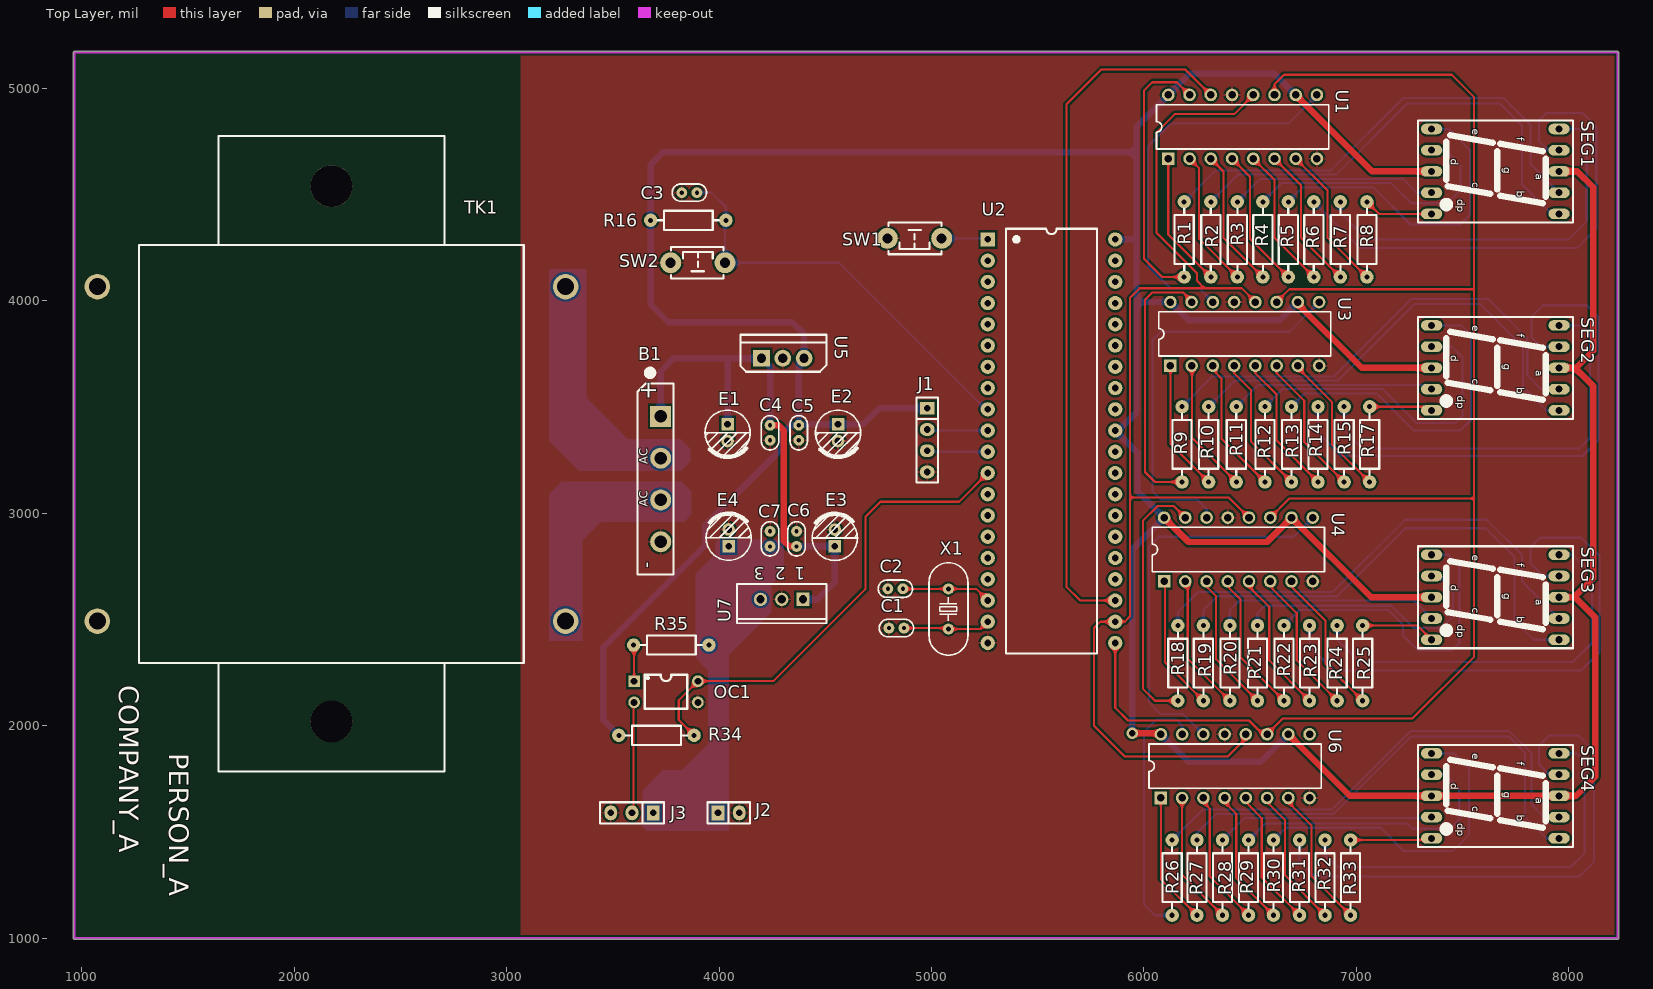
[diagram p0: Top Layer view]
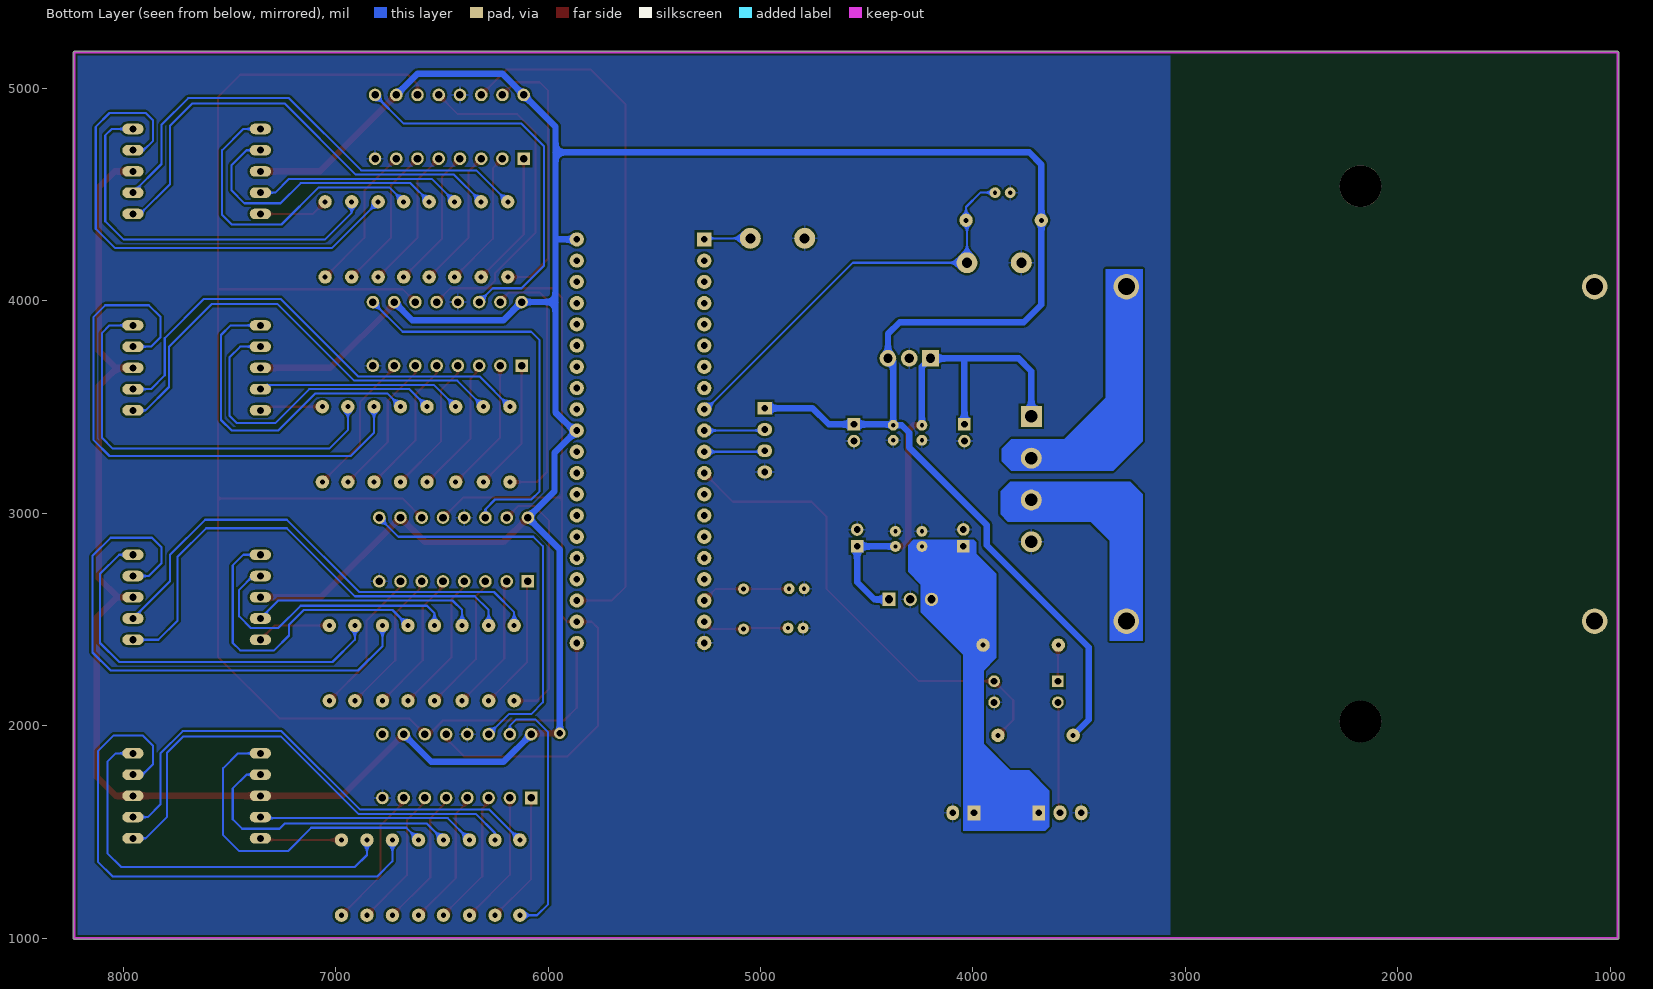
[diagram p1: Bottom Layer view, seen from below]
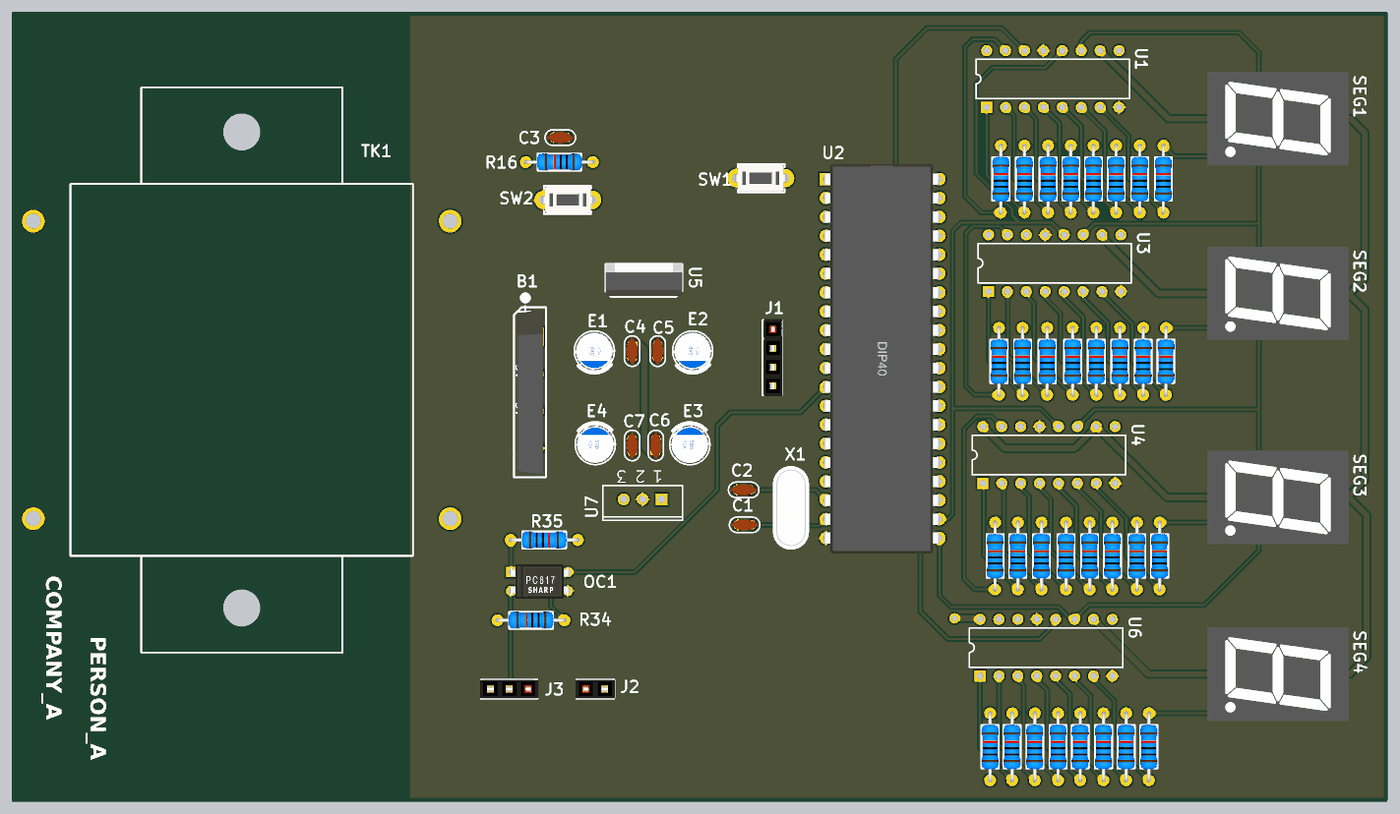
[diagram p2: 3D render of the assembled board from above, using the file's embedded part models]
# Altium PCB MISC84319.PcbDoc
Units mil, origin at the board's own origin, x right, y up, seen from the top; angles counter-clockwise.
Board outline 7275.03 x 4180.03 mil, 2 copper layers (Top Layer, Bottom Layer); 66 components, 85 nets, 271 pads, 1 vias.

## Layer stack, top to bottom (the 12.6 mil dielectric is the usual default, probably not edited)
Top Solder: solder mask 0.4, Solder Resist, Dk 3.5
Top Layer: signal copper 1.4
Dielectric 1: dielectric 12.6, FR-4, Dk 4.8
Bottom Layer: signal copper 1.4
Bottom Solder: solder mask 0.4, Solder Resist, Dk 3.5

## Board outline
965,994.99 cw(c965,1000) 959.99,1000 959.99,5170 cw(c965,5170) 965,5175.02 8230,5175.02 cw(c8230,5170) 8235.01,5170 8235.01,1000 cw(c8230,1000) 8230,994.99

## Design rules (kind name [scope] priority, off if disabled: settings)
Clearance [All] p1: gap=10
HoleSize [All] p1: absolutevalues=TRUE maxlimit=1000 minlimit=1 maxpercent=80.000 minpercent=20.000
MinimumSolderMaskSliver [All] p1: minsoldermaskwidth=0
PolygonConnect [All] p1: connectstyle=Relief reliefconductorwidth=10 reliefentries=4 polygonreliefangle="90 Angle" airgapwidth=10
RoutingVias [All] p1: holewidth=28 width=50 viastyle="Through Hole" minholewidth=28 minwidth=50 maxholewidth=28 maxwidth=50
SilkToSilkClearance [All] p1: silktosilkclearance=0
SilkToSolderMaskClearance [IsPad] p1: minsilkscreentomaskgap=0 clearancetoexposedcopper=TRUE
SolderMaskExpansion [All] p1: expansion=4
Width [All] p1: maxlimit=60 minlimit=10 preferedwidth=10
26 further rules are at their usual default settings.

## Components (designator, comment, footprint, x,y, rotation, side; value= is the part's Value field where it differs from the comment)
B1 "GBU" GBU 3725,3161.57 r90 top
C1 "1nF" "CC 1.8*3.6" 4835,2460 r0 top
C2 "1nF" "CC 1.8*3.6" 4830,2645 r0 top
C3 "100nF" "CC 1.8*3.6" 3860,4510 r0 top
C4 "1nF" "CC 1.8*3.6" 4240,3379.57 r90 top
C5 "1nF" "CC 1.8*3.6" 4375,3379.57 r90 top
C6 "1nF" "CC 1.8*3.6" 4365,2880 r270 top
C7 "1nF" "CC 1.8*3.6" 4240,2880 r270 top
E1 "220U" "CS 2.0*5*8 - C" 4040,3380 r90 top
E2 "220U" "CS 2.0*5*8 - C" 4560,3380 r90 top
E3 "220U" "CS 2.0*5*8 - C" 4545,2884.37 r270 top
E4 "220U" "CS 2.0*5*8 - C" 4045,2885 r270 top
J1 "Female HDR1X4" Fe-HDR1X4/2.54-S 4980,3495 r0 top
J2 "Female HDR1X2" Fe-HDR1X2/2.54-S 3995,1590 r0 top
J3 "Female HDR1X3" Fe-HDR1X3/2.54-S 3690,1590 r270 top
OC1 "PC817" DIP_PC817 3600,2210 r0 top
R1 "100R" "RS 1/4W" 6190,4290 r90 top
R2 "100R" "RS 1/4W" 6315,4290 r90 top
R3 "100R" "RS 1/4W" 6440,4290 r90 top
R4 "100R" "RS 1/4W" 6560,4290 r90 top
R5 "100R" "RS 1/4W" 6680,4290 r90 top
R6 "100R" "RS 1/4W" 6800,4290 r90 top
R7 "100R" "RS 1/4W" 6925,4290 r90 top
R8 "100R" "RS 1/4W" 7050,4290 r90 top
R9 "100R" "RS 1/4W" 6180,3325 r90 top
R10 "100R" "RS 1/4W" 6305,3325 r90 top
R11 "100R" "RS 1/4W" 6435,3325 r90 top
R12 "100R" "RS 1/4W" 6570,3325 r90 top
R13 "100R" "RS 1/4W" 6695,3325 r90 top
R14 "100R" "RS 1/4W" 6820,3325 r90 top
R15 "100R" "RS 1/4W" 6943.12,3325 r90 top
R16 "10K" "RS 1/4W" 3855,4380 r180 top
R17 "100R" "RS 1/4W" 7063.12,3325 r90 top
R18 "100R" "RS 1/4W" 6160,2295 r90 top
R19 "100R" "RS 1/4W" 6280,2295 r90 top
R20 "100R" "RS 1/4W" 6405,2295 r90 top
R21 "100R" "RS 1/4W" 6535,2295 r90 top
R22 "100R" "RS 1/4W" 6660,2295 r90 top
R23 "100R" "RS 1/4W" 6780,2295 r90 top
R24 "100R" "RS 1/4W" 6910,2295 r90 top
R25 "100R" "RS 1/4W" 7030,2295 r90 top
R26 "100R" "RS 1/4W" 6133.12,1285 r90 top
R27 "100R" "RS 1/4W" 6250,1285 r90 top
R28 "100R" "RS 1/4W" 6370,1285 r90 top
R29 "100R" "RS 1/4W" 6493.12,1285 r90 top
R30 "100R" "RS 1/4W" 6610,1285 r90 top
R31 "100R" "RS 1/4W" 6733.12,1285 r90 top
R32 "100R" "RS 1/4W" 6853.12,1285 r90 top
R33 "100R" "RS 1/4W" 6973.12,1285 r90 top
R34 "10K" "RS 1/4W" 3705,1955 r180 top
R35 "1K" "RS 1/4W" 3775,2380 r0 top
SEG1 "0.56IN-1-A" 0.56IN-1P 7355,4810 r270 top
SEG2 "0.56IN-1-A" 0.56IN-1P 7355,3885 r270 top
SEG3 "0.56IN-1-A" 0.56IN-1P 7355,2805 r270 top
SEG4 "0.56IN-1-A" 0.56IN-1P 7355,1870 r270 top
SW1 "3x6x5" "TSW DIP-3*6*5" 4920,4295 r180 top
SW2 "3x6x5" "TSW DIP-3*6*5" 3900,4180 r0 top
TK1 "TRAN-2P2S" TRANS2P2S 2175,3280 r90 top
U1 "SN74LS595" DIP-16 6465,4820 r0 top
U2 "AT89C51" DIP40 5565,3340 r0 top
U3 "SN74LS595" DIP-16 6475,3845 r0 top
U4 "SN74LS595" DIP-16 6445,2830 r0 top
U5 "LM7805" TO220A 4300,3730 r0 top
U6 "SN74LS595" DIP-16 6430,1810 r0 top
U7 "LM7812CT" T03B 4295,2595 r180 top
X1 "12MHz" "OSC HC-49S" 5080,2550 r270 top

## Footprints (in the part's own frame and the unit in brackets; to place one, negate y for a bottom-side part, rotate by r counter-clockwise, add the part's x,y. Pads: shape width x height; smd on the part's side, far side on the other; paste and mask are expansions set on the pad)
0.56IN-1P [mm]
  oval 1.27x2.54 hole 0.85: 1(0,0) 2(2.54,0) 3(5.08,0) 4(7.62,0) 5(10.16,0) 6(10.16,15.24) 7(7.62,15.24) 8(5.08,15.24) 9(2.54,15.24) 10(0,15.24)
  silkscreen extent -1.02,-1.65 11.18,16.89, body extent -1.22,-1.85 11.38,17.15, height 8
"CC 1.8*3.6" [mm] "脚距1.8mm直径3.6mm"
  round 1.3 hole 0.5: 1(-0.9,0) 2(0.9,0)
  silkscreen extent -2.05,-1.04 2.05,1.04, body extent -1.8,-0.8 1.8,0.8, height 3.6
"CS 2.0*5*8 - C" [mm] "脚距2mm , 直径5mm , 高8mm"
  rect 1.5x1.5 hole 0.8: 1(1,0)
  round 1.5 hole 0.8: 2(-1,0)
  silkscreen extent -2.96,-2.7 2.7,2.7, body extent -2.5,-2.5 2.5,2.5, height 8.02
DIP40 [mm]
  rect 1.7x1.7 hole 0.8: 1(-7.62,24.13)
  round 1.7 hole 0.8: 2(-7.62,21.59) 3(-7.62,19.05) 4(-7.62,16.51) 5(-7.62,13.97) 6(-7.62,11.43) 7(-7.62,8.89) 8(-7.62,6.35) 9(-7.62,3.81) 10(-7.62,1.27) 11(-7.62,-1.27) 12(-7.62,-3.81) 13(-7.62,-6.35) 14(-7.62,-8.89) 15(-7.62,-11.43) 16(-7.62,-13.97) 17(-7.62,-16.51) 18(-7.62,-19.05) 19(-7.62,-21.59) 20(-7.62,-24.13) 21(7.62,-24.13) 22(7.62,-21.59) 23(7.62,-19.05) 24(7.62,-16.51) 25(7.62,-13.97) 26(7.62,-11.43) 27(7.62,-8.89) 28(7.62,-6.35) 29(7.62,-3.81) 30(7.62,-1.27) 31(7.62,1.27) 32(7.62,3.81) 33(7.62,6.35) 34(7.62,8.89) 35(7.62,11.43) 36(7.62,13.97) 37(7.62,16.51) 38(7.62,19.05) 39(7.62,21.59) 40(7.62,24.13)
  silkscreen extent -5.46,-25.4 5.46,25.4, body extent -7.91,-26.19 7.65,26.16, height 4.7
DIP-16 [mm]
  rect 1.5x1.5 hole 0.9: 1(-8.89,-3.81)
  round 1.5 hole 0.9: 2(-6.35,-3.81) 3(-3.81,-3.81) 4(-1.27,-3.81) 5(1.27,-3.81) 6(3.81,-3.81) 7(6.35,-3.81) 8(8.89,-3.81) 9(8.89,3.81) 10(6.35,3.81) 11(3.81,3.81) 12(1.27,3.81) 13(-1.27,3.81) 14(-3.81,3.81) 15(-6.35,3.81) 16(-8.89,3.81)
  silkscreen extent -10.3,-2.65 10.3,2.65
DIP_PC817 [mm]
  rect 1.4x1.4 hole 0.813: 1(0,0)
  round 1.4 hole 0.813: 2(0,-2.54) 3(7.62,-2.54) 4(7.62,0)
  silkscreen extent 1.27,-3.3 6.35,0.76, body extent -0.13,-3.57 7.75,1.03, height 4.3
Fe-HDR1X2/2.54-S [mil] "Connector; Header; 2x2 Position"
  rect 60x70 hole 32: 1(0,0)
  oval 60x70 hole 32: 2(100,0)
  silkscreen extent -50,-50 150,50, body extent -55,-48 155,50, height 335
Fe-HDR1X3/2.54-S [mil]
  rect 70x60 hole 32: 1(0,0)
  oval 70x60 hole 32: 2(0,-100) 3(0,-200)
  silkscreen extent -50,-250 50,50, body extent -50,-255 48,55, height 335
Fe-HDR1X4/2.54-S [mil]
  rect 70x60 hole 32: 1(0,0)
  oval 70x60 hole 32: 2(0,-100) 3(0,-200) 4(0,-300)
  silkscreen extent -50,-350 50,50, body extent -44,-355 54,55, height 335
GBU [mm] "整流桥，脚距：5mm/200mil"
  round 2.5 hole 1.5: AC1(-2.5,0) AC2(2.5,0) DC-(-7.5,0)
  rect 2.5x2.5 hole 1.5: DC+(7.5,0)
  silkscreen extent -11.43,-1.52 13.06,2.79, body extent -11,-1.15 11,2.35, height 20.8
"OSC HC-49S" [mm]
  round 1.3 hole 0.6: 1(-2.4,0) 2(2.4,0)
  silkscreen extent -5.52,-2.32 5.52,2.33, body extent -5.52,-2.32 5.53,2.33, height 4.13
"RS 1/4W" [mm] "直插色环电阻，脚距9mm，直径2.3mm"
  round 1.6 hole 0.6: 1(-4.5,0) 2(4.5,0)
  silkscreen extent -3.68,-1.14 3.68,1.14, body extent -4.72,-1.16 4.73,1.16, height 2.32
T03B [mm] "TO, Thru-Hole, Vertical, Heatsink Mounted; 3 In-Line Leads; Pitch 2.54 mm"
  rect 1.6x1.6 hole 1: 1(-2.54,0)
  round 1.6 hole 1: 2(0,0) 3(2.54,0)
  silkscreen extent -5.35,-1.85 5.35,2.85
TO220A [mm] "220，3脚晶体管"
  rect 2x2 hole 1.1: 1(-2.54,0)
  round 2 hole 1.1: 2(0,0) 3(2.54,0)
  silkscreen extent -5.08,-1.6 5.21,2.82, body extent -5.08,-1.45 5.22,2.98, height 18.5
TRANS2P2S [mil]
  round 120 hole 80 paste+4 mask+4: 1(-787.4,1102.36) 2(787.4,1102.36) 3(-787.4,-1102.36) 4(787.4,-1102.36)
  round 196.85 hole 196.85 unplated paste+0: ""(-1259.84,0) ""(1259.84,0)
  silkscreen extent -1496,-906 1496,906
"TSW DIP-3*6*5" [mm] "3*6*5mm"
  round 2.5 hole 1.2: 1(3.25,0) 2(-3.25,0)
  silkscreen extent -3.21,-1.9 3.09,1.9, body extent -3.91,-1.75 3.91,1.75, height 5.01

## Part data
B1: "1kV/10A bridge rectifier"
C1 C2 C3 C4 C5 C6 C7: library part CC, "ceramic disc capacitor"
E1 E2 E3 E4: library part CS, "through-hole solid-state capacitor"
OC1: "linear optocoupler"
R1 R2 R3 R4 R5 R6 R7 R8 R9 R10 R11 R12 R13 R14 R15 R16 R17 R18 R19 R20 R21 R22 R23 R24 R25 R26 R27 R28 R29 R30 R31 R32 R33 R34 R35: library part R-S, "colour-band resistor"
SEG1 SEG2 SEG3 SEG4: "1-digit 0.56 inch common-anode display"
SW1 SW2: library part "TSW 3x6", "3x6 tact switch"
U1 U3 U4 U6: "8-BIT SFT REG WIRTH OUTPUT LCH"
U2: library part STC89C51
U7: "Series 3-Terminal Positive Regulator"
X1: library part XTAL-2P, "2-pin passive crystal oscillator"

## Via types
v1: diameter 55.12, hole 31.5, Top Layer to Bottom Layer, 1 vias

## Nets (pads, with @x,y where several pads share a name; then routed paths per layer and width w, separated by ;. In a path a pad name is that pad's centre, name@x,y a point inside that pad or via, vN(x,y) a via of type N, cw(c..) or ccw(c..) an arc to the next point about the centre after c; other vN are vias at no path point)
+12V: C7.2 E4.1 J2.1 J3.1 R35.2 U7.3 | length 1.5
  Bottom Layer w60: C7.2@4238.94,2845.63 C7.2
GND: B1.DC- C1.1 C2.1 C3.1 C4.1 C5.1 C6.1 C7.1 E1.2 E2.2 E3.2 E4.2 J1.4 J2.2 J3.3 OC1.3 SW1.1 SW2.2 U1.8 U1.13 U2.20 U3.8 U3.13 U4.8 U4.13 U5.2 U6.8 U6.13 U7.2
NetB1_AC1: B1.AC1 TK1.3
NetB1_AC2: B1.AC2 TK1.4
NetB1_DC+: B1.DC+ C4.2 C6.2 E1.1 E3.1 U5.1 U7.1 | length 2557.2
  Top Layer w30: C4.2 4280,3415 4305,3390 4305,2870 4330.43,2844.57 C6.2
  Bottom Layer w30: B1.DC+ 3725,3670 3785,3730 4035,3730 ; E1.1 4040,3725 4035,3730 ; C4.2 4240,3690 U5.1 4035,3730 ; C6.2@4364.32,2844.57 C6.2 4544.57,2844.57 E3.1 4545,2675 4465,2595 U7.1
NetC1_2: C1.2 U2.19 X1.2 | length 410.7
  Top Layer w10: C1.2 5075.51,2460 X1.2 5230.51,2455.51 U2.19
NetC2_2: C2.2 U2.18 X1.1 | length 422.3
  Top Layer w10: C2.2 4865.94,2644.49 X1.1 5210.51,2644.49 U2.18
NetC3_2: C3.2 R16.1 SW2.1 U2.9 | length 1952
  Bottom Layer w10: C3.2 3965,4510 4032.17,4442.83 R16.1 4027.95,4375.79 SW2.1 4565,4180 5255,3490 U2.9
NetJ3_2: J3.2 OC1.2 | length 524.1
  Top Layer w10: J3.2 3597.05,1597.05 3597.05,2107.05 OC1.2
NetOC1_1: OC1.1 R35.1 | length 170.9
  Top Layer w10: R35.1 3600,2377.83 OC1.1
NetR1_1: R1.1 U1.15 | length 1272.5
  Top Layer w10: R1.1 6087.17,4112.83 6000,4200 6000,4990 6040,5030 6155,5030 U1.15
NetR1_2: R1.2 SEG1.7 | length 2259.8
  Bottom Layer w10: R1.2 6337.83,4615 6880,4615 7220,4955 7695,4955 7820,4830 7820,4645 SEG1.7
NetR2_1: R2.1 U1.1 | length 640
  Top Layer w10: U1.1 6115,4312.83 R2.1
NetR2_2: R2.2 SEG1.6 | length 2208.2
  Bottom Layer w10: R2.2 6442.83,4595 6905,4595 7240,4930 7675,4930 7780,4825 7780,4550 7920,4410 SEG1.6
NetR3_1: R3.1 U1.2 | length 650.4
  Top Layer w10: U1.2 6260,4625 6260,4292.83 R3.1
NetR3_2: R3.2 SEG1.4 | length 986.6
  Bottom Layer w10: R3.2 6547.83,4575 7220,4575 7285,4510 SEG1.4
NetR4_1: R4.1 U1.3 | length 658.6
  Top Layer w10: U1.3 6375,4610 6375,4297.83 R4.1
NetR4_2: R4.2 SEG1.2 | length 1314.6
  Bottom Layer w10: R4.2 6647.83,4555 7165,4555 7260,4460 7430,4460 7490,4520 7490,4640 7420,4710 SEG1.2
NetR5_1: R5.1 U1.4 | length 666.9
  Top Layer w10: U1.4 6500,4585 6500,4292.83 R5.1
NetR5_2: R5.2 SEG1.1 | length 1500.6
  Bottom Layer w10: R5.2 6747.83,4535 7080,4535 7255,4360 7490,4360 7535,4405 7535,4710 7435,4810 SEG1.1
NetR6_1: R6.1 U1.5 | length 675.2
  Top Layer w10: U1.5 6615,4570 6615,4297.83 R6.1
NetR6_2: R6.2 SEG1.9 | length 2457.3
  Bottom Layer w10: R6.2 7017.17,4250 8040,4250 8130,4340 8130,4820 8065,4885 7895,4885 7860,4850 7860,4755 7905,4710 SEG1.9
NetR7_1: R7.1 U1.6 | length 685.6
  Top Layer w10: U1.6 6740,4545 6740,4297.83 R7.1
NetR7_2: R7.2 SEG1.10 | length 1846.6
  Bottom Layer w10: R7.2 6925,4415 7050,4290 8000,4290 8085,4375 8085,4780 8055,4810 SEG1.10
NetR8_1: R8.1 U1.7 | length 695.9
  Top Layer w10: U1.7 6865,4520 6865,4297.83 R8.1
NetR8_2: R8.2 SEG1.5 | length 328.7
  Top Layer w10: R8.2 7107.17,4410 SEG1.5
NetR9_1: R9.1 U3.15 | length 1260.6
  Top Layer w10: R9.1 6052.17,3147.83 6005,3195 6005,4005 6040,4040 6185,4040 6225,4000 U3.15
NetR9_2: R9.2 SEG2.7 | length 2263.9
  Bottom Layer w10: R9.2 6322.83,3645 6895,3645 7260,4010 7620,4010 7805,3825 7805,3650 7870,3585 SEG2.7
NetR10_1: R10.1 U3.1 | length 601.7
  Top Layer w10: U3.1@6125,3675 6125,3327.83 R10.1
NetR10_2: R10.2 SEG2.6 | length 2168.4
  Bottom Layer w10: R10.2 6427.83,3625 6913.28,3625 7273.28,3985 7585,3985 7785,3785 7785,3595 7895,3485 SEG2.6
NetR11_1: R11.1 U3.2 | length 614.2
  Top Layer w10: U3.2@6225,3675 6226.5,3673.5 6226.5,3356.34 R11.1
NetR11_2: R11.2 SEG2.4 | length 970.9
  Bottom Layer w10: R11.2 6537.83,3605 7335,3605 SEG2.4
NetR12_1: R12.1 U3.3 | length 648.6
  Top Layer w10: U3.3 6340,3680 6340,3660 6365,3635 6365,3352.83 R12.1
NetR12_2: R12.2 SEG2.2 | length 1485.8
  Bottom Layer w10: R12.2 6652.83,3585 7125,3585 7285,3425 7465,3425 7500,3460 7500,3735 7450,3785 SEG2.2
NetR13_1: R13.1 U3.4 | length 659
  Top Layer w10: U3.4 6425,3660 6505,3580 6505,3337.83 R13.1
NetR13_2: R13.2 SEG2.1 | length 1567.9
  Bottom Layer w10: R13.2 6757.83,3565 7095,3565 7270,3390 7490,3390 7540,3440 7540,3840 7495,3885 SEG2.1
NetR14_1: R14.1 U3.5 | length 669.4
  Top Layer w10: U3.5 6525,3660 6625,3560 6625,3342.83 R14.1
NetR14_2: R14.2 SEG2.9 | length 2703
  Bottom Layer w10: R14.2 6820,3380 6930,3270 8065,3270 8140,3345 8140,3925 8085,3980 7880,3980 7825,3925 7825,3830 7870,3785 SEG2.9
NetR15_1: R15.1 U3.6 | length 678.9
  Top Layer w10: U3.6 6625,3660 6755,3530 6755,3335.95 R15.1
NetR15_2: R15.2 SEG2.10 | length 1978.4
  Bottom Layer w10: R15.2 6943.12,3391.88 7030,3305 8050,3305 8100,3355 8100,3850 8065,3885 SEG2.10
NetR17_1: R17.1 U3.7 | length 701.4
  Top Layer w10: U3.7 6715,3695 6885,3525 6885,3325.95 R17.1
NetR17_2: R17.2 SEG2.5 | length 299
  Top Layer w10: R17.2 7337.83,3502.17 SEG2.5
NetR18_1: R18.1 U4.15 | length 1255.2
  Top Layer w10: R18.1 6052.17,2117.83 5995,2175 5995,2965 6065,3035 6140,3035 U4.15 U4.15@6212.5,2962.5
NetR18_2: R18.2 SEG3.7 | length 2303.9
  Bottom Layer w10: R18.2 6160,2535 6255,2630 6890,2630 7230,2970 7615,2970 7780,2805 7780,2680 SEG3.7
NetR19_1: R19.1 U4.1 | length 606.7
  Top Layer w10: 6100,2650 6100,2297.83 R19.1
NetR19_2: R19.2 SEG3.6 | length 2300.5
  Bottom Layer w10: R19.2 6280,2545 6345,2610 6910,2610 7230,2930 7610,2930 7745,2795 7745,2495 7835,2405 SEG3.6
NetR20_1: R20.1 U4.2 | length 649.2
  Top Layer w10: U4.2 6206.5,2668.5 6206.5,2316.34 R20.1
NetR20_2: R20.2 SEG3.4 | length 1076.7
  Bottom Layer w10: R20.2 6405,2545 6450,2590 7270,2590 SEG3.4
NetR21_1: R21.1 U4.3 | length 661.6
  Top Layer w10: U4.3 6300,2675 6300,2650 6340,2610 6340,2312.83 R21.1
NetR21_2: R21.2 SEG3.2 | length 1310.5
  Bottom Layer w10: R21.2 6535,2530 6570,2565 7165,2565 7270,2460 7400,2460 7455,2515 7455,2640 7390,2705 SEG3.2
NetR22_1: R22.1 U4.4 | length 671.9
  Top Layer w10: U4.4 6400,2675 6400,2650 6455,2595 6455,2322.83 R22.1
NetR22_2: R22.2 SEG3.1 | length 1493.4
  Bottom Layer w10: R22.2 6732.83,2545 7150,2545 7220,2475 7220,2425 7290,2355 7450,2355 7485,2390 7485,2755 7435,2805 SEG3.1
NetR23_1: R23.1 U4.5 | length 680.2
  Top Layer w10: U4.5 6495,2655 6590,2560 6590,2307.83 R23.1
NetR23_2: R23.2 SEG3.9 | length 2613.7
  Bottom Layer w10: R23.2 6780,2375 6895,2260 8060,2260 8145,2345 8145,2800 8060,2885 7865,2885 7820,2840 7820,2765 7880,2705 SEG3.9
NetR24_1: R24.1 U4.6 | length 692.6
  Top Layer w10: U4.6 6605,2670 6605,2645 6720,2530 6720,2307.83 R24.1
NetR24_2: R24.2 SEG3.10 | length 1865.2
  Bottom Layer w10: R24.2 6910,2405 7015,2300 8020,2300 8110,2390 8110,2715 8020,2805 SEG3.10
NetR25_1: R25.1 U4.7 | length 700.9
  Top Layer w10: U4.7 6700,2675 6700,2650 6855,2495 6855,2292.83 R25.1
NetR25_2: R25.2 SEG3.5 | length 352.8
  Top Layer w10: R25.2 7287.83,2472.17 SEG3.5
NetR26_1: R26.1 U6.15 | length 1222
  Bottom Layer w10: R26.1 6052.17,1107.83 6000,1160 6000,1970 6060,2030 6150,2030 6180,2000 U6.15
NetR26_2: R26.2 SEG4.7 | length 2342.6
  Bottom Layer w10: R26.2 6275.95,1605 6885,1605 7255,1975 7720,1975 7825,1870 7825,1630 7885,1570 SEG4.7
NetR27_1: R27.1 U6.1 | length 602.6
  Top Layer w10: U6.1@6080,1640 6080,1277.83 R27.1
NetR27_2: R27.2 SEG4.6 | length 2301.9
  Bottom Layer w10: R27.2 6250,1495 6340,1585 6893.28,1585 7258.28,1950 7716.72,1950 7795,1871.72 7795,1570 7895,1470 SEG4.6
NetR28_1: R28.1 U6.2 | length 610.9
  Top Layer w10: U6.2@6180,1640 6180,1297.83 R28.1
NetR28_2: R28.2 SEG4.4 | length 1029.7
  Bottom Layer w10: R28.2 6472.83,1565 7350,1565 SEG4.4
NetR29_1: R29.1 U6.3 | length 620.4
  Top Layer w10: U6.3@6280,1640 6310,1610 6310,1290.95 R29.1
NetR29_2: R29.2 SEG4.2 | length 1355
  Bottom Layer w10: R29.2 6570.95,1540 7240,1540 7265,1515 7440,1515 7485,1560 7485,1705 7420,1770 SEG4.2
NetR30_1: R30.1 U6.4 | length 627.4
  Top Layer w10: U6.4@6380,1640 6435,1585 6435,1282.83 R30.1
NetR30_2: R30.2 SEG4.1 | length 1539.6
  Bottom Layer w10: R30.2 6667.83,1520 7115,1520 7225,1410 7455,1410 7530,1485 7530,1800 7460,1870 SEG4.1
NetR31_1: R31.1 U6.5 | length 657
  Top Layer w10: U6.5 6490,1650 6490,1630 6555,1565 6555,1285.95 R31.1
NetR31_2: R31.2 SEG4.9 | length 2578.4
  Bottom Layer w10: R31.2 6733.12,1361.88 6805,1290 8050,1290 8120,1360 8120,1880 8045,1955 7910,1955 7860,1905 7860,1820 7910,1770 SEG4.9
NetR32_1: R32.1 U6.6 | length 665.3
  Top Layer w10: U6.6 6590,1650 6590,1630 6665,1555 6665,1295.95 R32.1
NetR32_2: R32.2 SEG4.10 | length 1909.2
  Bottom Layer w10: R32.2 6853.12,1391.88 6910,1335 8010,1335 8075,1400 8075,1830 8035,1870 SEG4.10
NetR33_1: R33.1 U6.7 | length 673.6
  Top Layer w10: U6.7 6680,1640 6790,1530 6790,1290.95 R33.1
NetR33_2: R33.2 SEG4.5 | length 385.1
  Top Layer w10: R33.2 7347.17,1462.17 SEG4.5
NetSW1_2: SW1.2 U2.1 | length 219.1
  Bottom Layer w10: SW1.2 5260,4295 U2.1
NetU1_9: U1.9 U3.14 | length 1834.8
  Bottom Layer w10: U3.14 6260,4060 6125,4060 6020,4165 6020,4730 6125,4835 6680,4835 U1.9
NetU1_11: U1.11 U2.21 U3.11 U4.11 U6.11 | length 7847.6
  Top Layer w10: U2.21 5865,2085 5925,2025 6495,2025 U6.11@6580,1940 ; U6.11 6655,2035 7265,2035 7555,2325 7555,3070 ; U4.11 6685,3070 7555,3070 ; U1.11 6615,5020 6660,5065 7450,5065 7555,4960 7555,4060 ; U3.11 6685,4055 7550,4055 7555,4060 ; 7555,3070 7555,4060
NetU1_12: U1.12 U2.22 U3.12 U4.12 U6.12 | length 5553.7
  Top Layer w10: U6.12@6480,1940 6395,1855 5910,1855 5765,2000 5765,2460 5795,2490 U2.22 5910,2490 5935,2515 5935,3075 ; U4.12 6400,3075 5935,3075 ; U1.12 6425,4880 6145,4880 6060,4795 6060,4320 6250,4130 6250,4095 6285,4060 ; U3.12 6460,4060 6285,4060 ; 5935,3075 5935,4015 5980,4060 6285,4060
NetU1_14: U1.14 U2.23 | length 3325
  Top Layer w10: U2.23 5700,2590 5635,2655 5635,4925 5800,5090 6195,5090 U1.14
NetU3_9: U3.9 U4.14 | length 1899.8
  Bottom Layer w10: U4.14 6295,3020 6250,3065 6080,3065 6040,3105 6040,3815 6080,3855 6685,3855 U3.9
NetU4_9: U4.9 U6.14 | length 1878.1
  Bottom Layer w10: U6.14 6185,2055 6080,2055 6025,2110 6025,2845 6070,2890 6705,2890 U4.9
P3.2: OC1.4 R34.1 U2.12 | length 2292.3
  Top Layer w10: R34.1 3810,2027.17 3810,2120 OC1.4 4255,2210 4690,2645 4690,2985 4760,3055 5130,3055 U2.12
RXD: J1.3 U2.11 | length 287.1
  Bottom Layer w10: J1.3 4985,3290 U2.11
TXD: J1.2 U2.10 | length 287.1
  Bottom Layer w10: J1.2 4985,3390 U2.10
VCC: C5.2 E2.1 J1.1 R16.2 R34.2 SEG1.3 SEG1.8 SEG2.3 SEG2.8 SEG3.3 SEG3.8 SEG4.3 SEG4.8 U1.10 U1.16 U2.31 U2.40 U3.10 U3.16 U4.10 U4.16 U5.3 U6.10 U6.16 | length 20390.9
  Top Layer w30: v1(5945,1965) 6075,1965 U6.16 ; U4.16 6210,2865 6580,2865 U4.10 7070,2605 SEG3.3 ; U6.10 6970,1670 SEG4.3 SEG4.8 8035,1670 8125,1760 8125,2510 8030,2605 8025,2605 ; U1.10 7075,4610 SEG1.3 ; U3.10 6725,3985 7025,3685 SEG2.3 ; SEG3.8 8025,2605 ; SEG2.8 8030,3685 ; SEG1.8 8040,4610 8115,4535 8115,3765 8035,3685 8030,3685 ; 8025,2605 8115,2695 8115,3600 8030,3685
  Bottom Layer w30: R34.2 3455,2027.83 3455,2370 3935,2850 3935,2945 4300,3310 4300,3380 4335,3415 C5.2 ; J1.1 4755,3495 4679.37,3419.37 E2.1 4379.37,3419.37 C5.2 ; U2.40 5960,4290 5965,4295 ; v1(5945,1965) 5945,2830 U4.16 5970,3105 5970,3285 U2.31 5880,3390 5965,3475 5965,3995 ; U6.16 6210,1830 6550,1830 U6.10 ; U1.10 6615,5070 6215,5070 U1.16 5965,4820 5965,4700 ; U3.10 6640,3910 6210,3910 U3.16 5965,3995 ; C5.2 4375,3705 U5.3 4400,3845 4345,3900 3760,3900 3677.83,3982.17 R16.2 3677.83,4642.83 3735,4700 5965,4700 ; 5965,3995 5965,4295 ; 5965,4295 5965,4700
pads on no net: TK1. TK1.1 TK1.2 U2.2 U2.3 U2.4 U2.5 U2.6 U2.7 U2.8 U2.13 U2.14 U2.15 U2.16 U2.17 U2.24 U2.25 U2.26 U2.27 U2.28 U2.29 U2.30 U2.32 U2.33 U2.34 U2.35 U2.36 U2.37 U2.38 U2.39 U6.9

## Polygon pours and split planes (outlines as drawn)
GND on Top Layer "D" (solid, remove dead copper, pour order 8): 2855,5690 2895,5730 8475,5730 8475,460 8720,215 8285,650 425,650 425,5770 305,5890
GND on Bottom Layer "D" (solid, remove dead copper, pour order 10): 700,5695 940,5935 9040,5935 9040,615 8645,220 8320,545 580,545

## Keep-outs
Keep-Out Layer:
  lines w10: 6850,5170 8230,5170 8230,5015 ; 6860,5170 965,5170 965,1000 8230,1000 8230,5080

## Other copper
Top Layer:
  pour cut-out: 965,5170 3065,5170 3065,1000 965,1000
Bottom Layer:
  region net NetB1_AC1: 3200,2400 3355,2400 3355,2870 3445,2960 3835,2960 3870,2995 3870,3105 3825,3150 3260,3150 3200,3090
  region net NetB1_AC2: 3200,4150 3375,4150 3375,3545 3570,3350 3820,3350 3865,3305 3865,3245 3820,3200 3340,3200 3200,3340
  region net +12V: 4280,2875 4305,2850 4305,2725 4245,2665 4245,2535 4045,2335 4045,1505 3660,1505 3640,1525 3640,1695 3735,1790 3825,1790 3950,1915 3950,2260 3890,2320 3890,2715 3985,2810 3985,2865 3995,2875
  pour cut-out: 965,5170 3070,5170 3070,1000 965,1000

## Silkscreen, mask and mechanical layers (free items; w line width, h text height)
Top Overlay:
  text "COMPANY_A" at 1145,2190 h160 r270
  text "PERSON_A" at 1380,1870 h160 r270